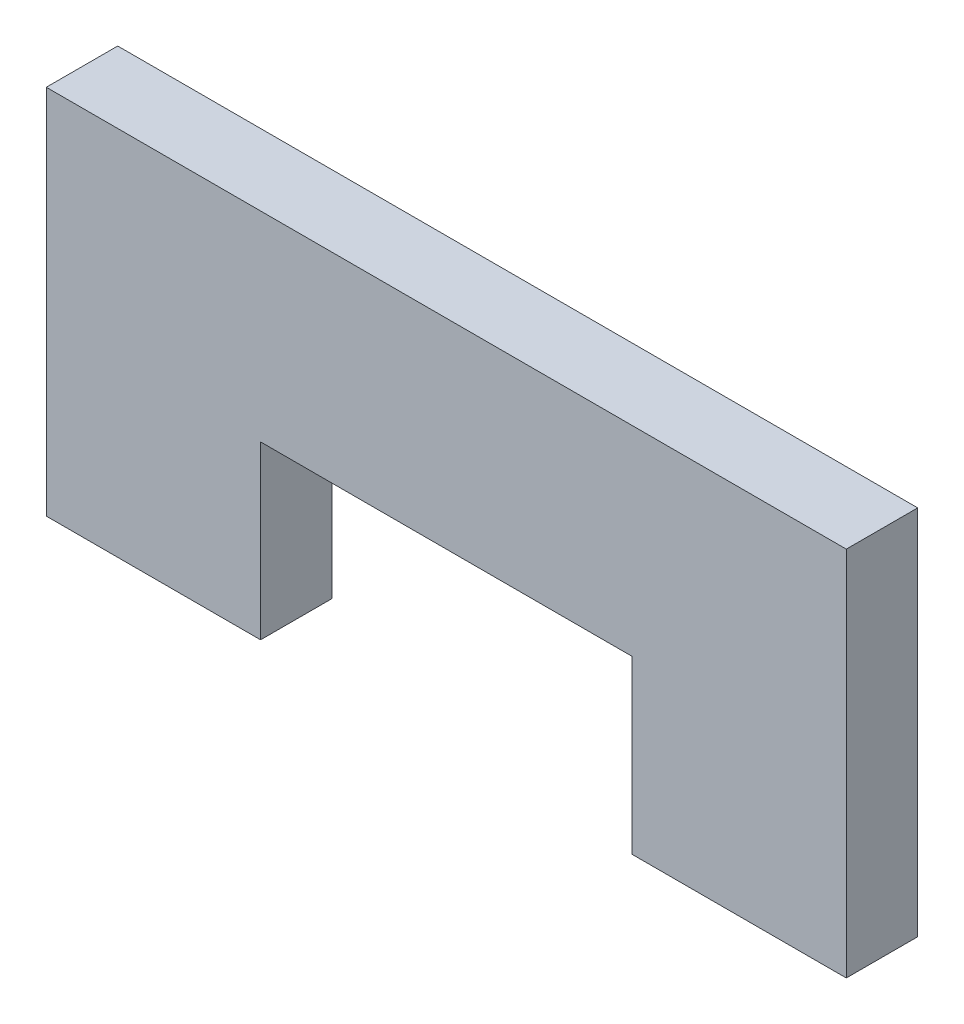
SolidWorks part; units mm, degrees
ref_plane "Front Plane" through (0, 0, 0) normal (0, 0, 1) x (1, 0, 0)
ref_plane "Top Plane" through (0, 0, 0) normal (0, 1, 0) x (1, 0, 0)
ref_plane "Right Plane" through (0, 0, 0) normal (1, 0, 0) x (0, 0, -1)
sketch "Sketch1" plane through (0, 0, 0) normal (0, 0, 1) x (1, 0, 0)
  line L0 (0, 0) -> (0, -97.858) construction
  line L1 (-140, 65) -> (140, 65)
  line L2 (-140, 65) -> (-140, -65)
  line L3 (-140, -65) -> (-65, -65)
  line L4 (140, 65) -> (140, -65)
  line L5 (-140, 65) -> (140, -65) construction
  line L6 (-140, -65) -> (140, 65) construction
  line L7 (-65, -5) -> (65, -5)
  line L8 (-65, -5) -> (-65, -65)
  line L10 (65, -5) -> (65, -65)
  line L11 (-65, -5) -> (65, -65) construction
  line L12 (-65, -65) -> (65, -5) construction
  line L13 (65, -65) -> (140, -65)
  point P0 (0, 0)
  point P6 (0, -35)
  dimension "D1" = 130
  dimension "D2" = 60
  dimension "D3" = 280
  dimension "D4" = 130
extrude "Boss-Extrude1" add sketch "Sketch1" along normal blind 25
